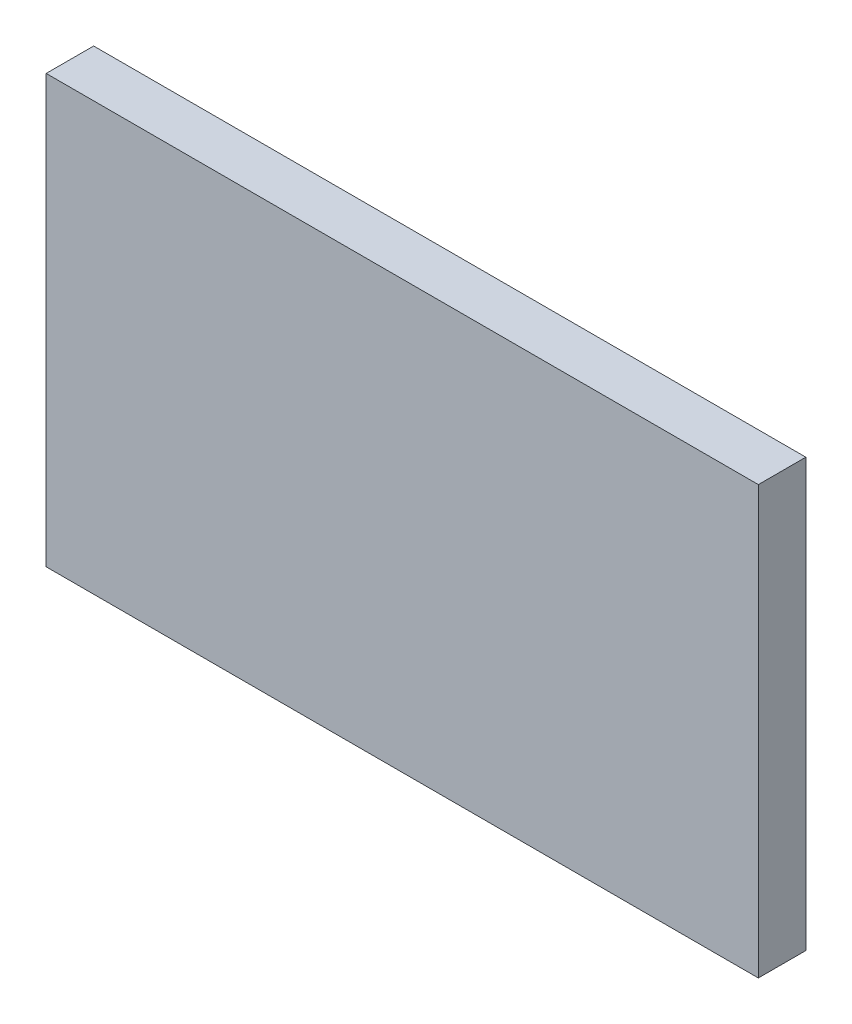
SolidWorks part; units mm, degrees
ref_plane "前视基准面" through (0, 0, 0) normal (0, 0, 1) x (1, 0, 0)
ref_plane "上视基准面" through (0, 0, 0) normal (0, 1, 0) x (1, 0, 0)
ref_plane "右视基准面" through (0, 0, 0) normal (1, 0, 0) x (0, 0, -1)
sketch "草图1" plane through (0, 0, 0) normal (0, 0, 1) x (1, 0, 0)
  line L0 (0, 0) -> (150, 0)
  line L1 (150, 0) -> (150, 90)
  line L2 (150, 90) -> (0, 90)
  line L3 (0, 90) -> (0, 0)
extrude "凸台-拉伸1" add sketch "草图1" along normal blind 10
